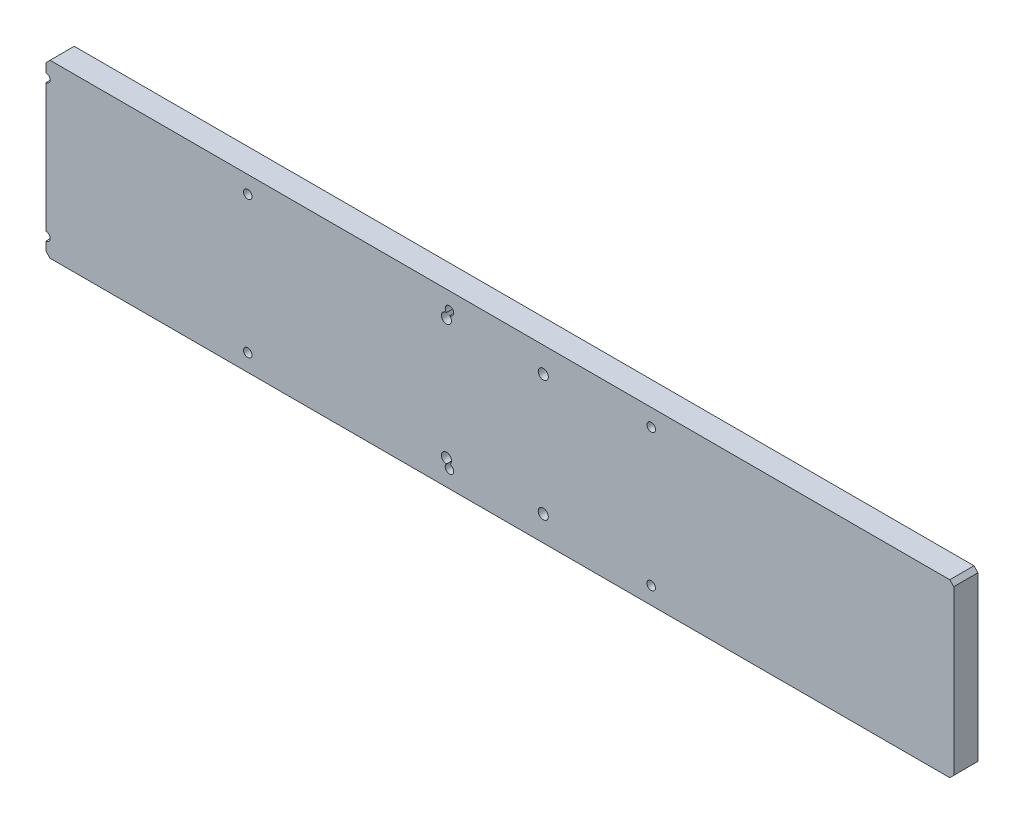
from build123d import *

# Parameters (mm, degrees)
SKETCH_1_W         = 450
SKETCH_1_H         = 85
EXTRUDE_1_DEPTH    = 12
HOLE_WIZARD_M6_1_D = 5
HOLE_WIZARD_M5_1_D = 4.2
F_5_0MM_1_D        = 5
F_5_0MM_1_DEPTH    = 5
F_5_0MM_1_TIP      = 1.502151548
CHAMFER_1_SIZE     = 2


with BuildPart() as part:
    # 草图1 → 凸台-拉伸1 (new body)
    with BuildSketch(Plane.XY):
        Rectangle(SKETCH_1_W, SKETCH_1_H)
    extrude(amount=EXTRUDE_1_DEPTH)

    # M6 螺纹孔1 (through all)
    with Locations(Plane(origin=(0, 0, 0), x_dir=(-1, 0, 0), z_dir=(0, 0, -1))):
        with Locations((26.5, 30), (-21.5, -30), (-21.5, 30), (26.5, -30), (-253.5, 30), (-301.5, -30), (-301.5, 30), (-253.5, -30)):
            Hole(HOLE_WIZARD_M6_1_D / 2)

    # M5 螺纹孔1 (through all)
    with Locations(Plane.XY.offset(12)):
        with Locations((75, 34), (75, -34), (-25, 34), (-25, -34), (-125, 34), (-125, -34), (-225, 34), (-225, -34)):
            Hole(HOLE_WIZARD_M5_1_D / 2)

    # Ø5.0mm 暗销孔1
    with Locations(Plane(origin=(0, 0, 0), x_dir=(-1, 0, 0), z_dir=(0, 0, -1))):
        with Locations((-75, 0), (225, 0)):
            Hole(F_5_0MM_1_D / 2, depth=F_5_0MM_1_DEPTH)
            with Locations((0, 0, -(F_5_0MM_1_DEPTH + F_5_0MM_1_TIP / 2))):  # 118° drill point
                Cone(0, F_5_0MM_1_D / 2, F_5_0MM_1_TIP, mode=Mode.SUBTRACT)

    # 倒角1
    chamfer_1_edges = [part.edges().sort_by_distance(p)[0] for p in [
        (225, -42.5, 6),
        (-225, -42.5, 6),
        (-225, 42.5, 6),
        (225, 42.5, 6),
    ]]
    chamfer(chamfer_1_edges, length=CHAMFER_1_SIZE)


solid = part.part
